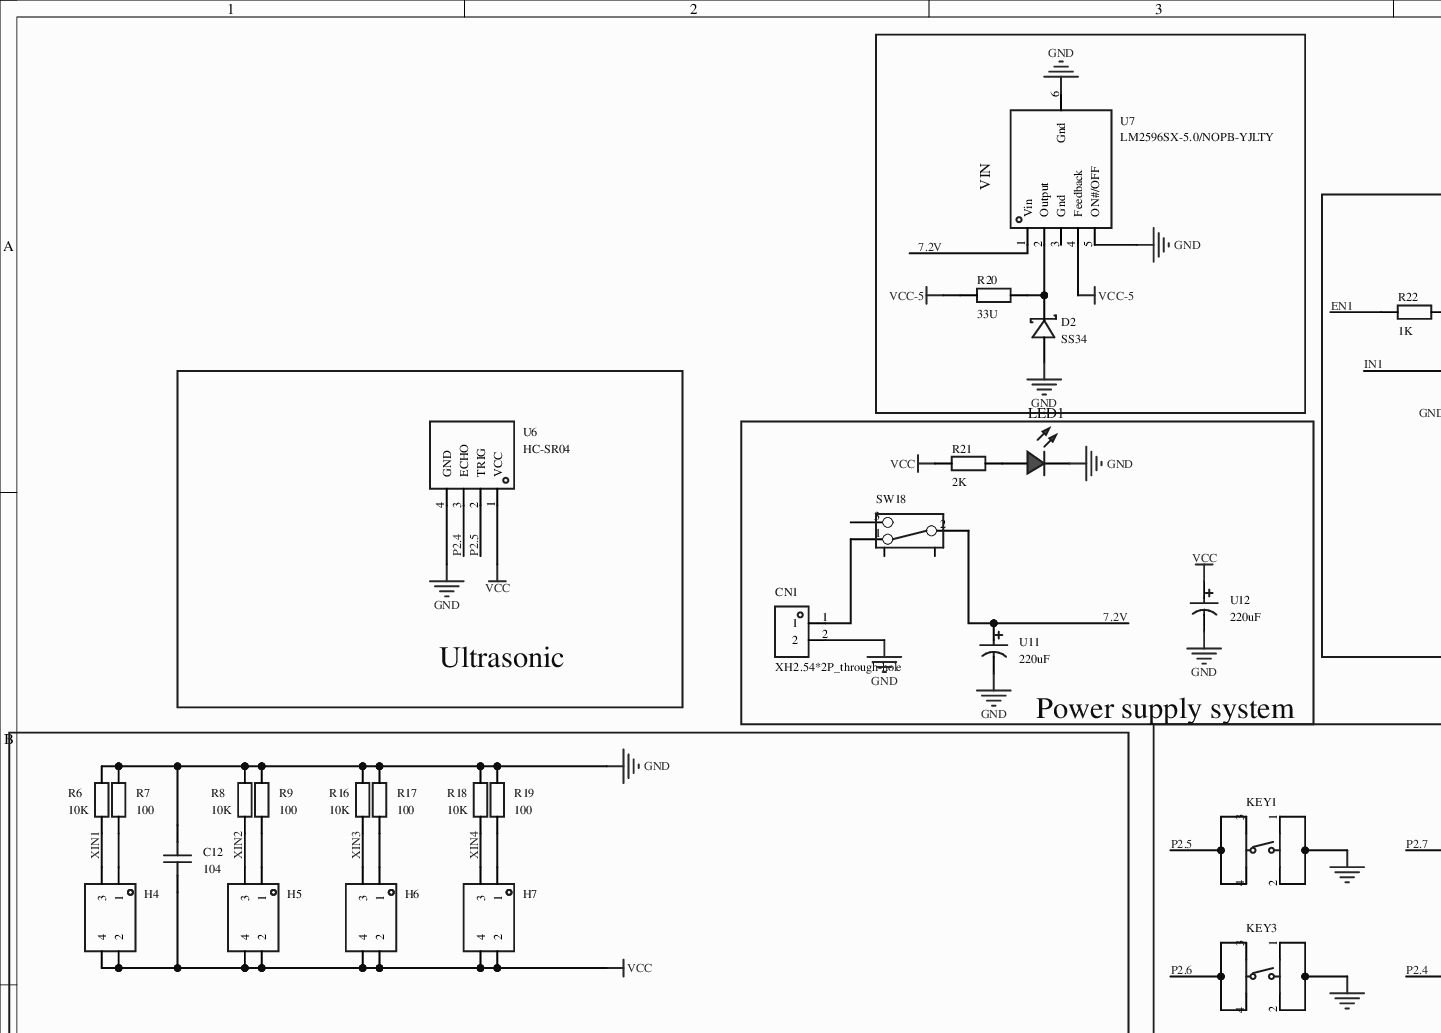
[diagram p0: MISC51732-3.schdoc, top left]
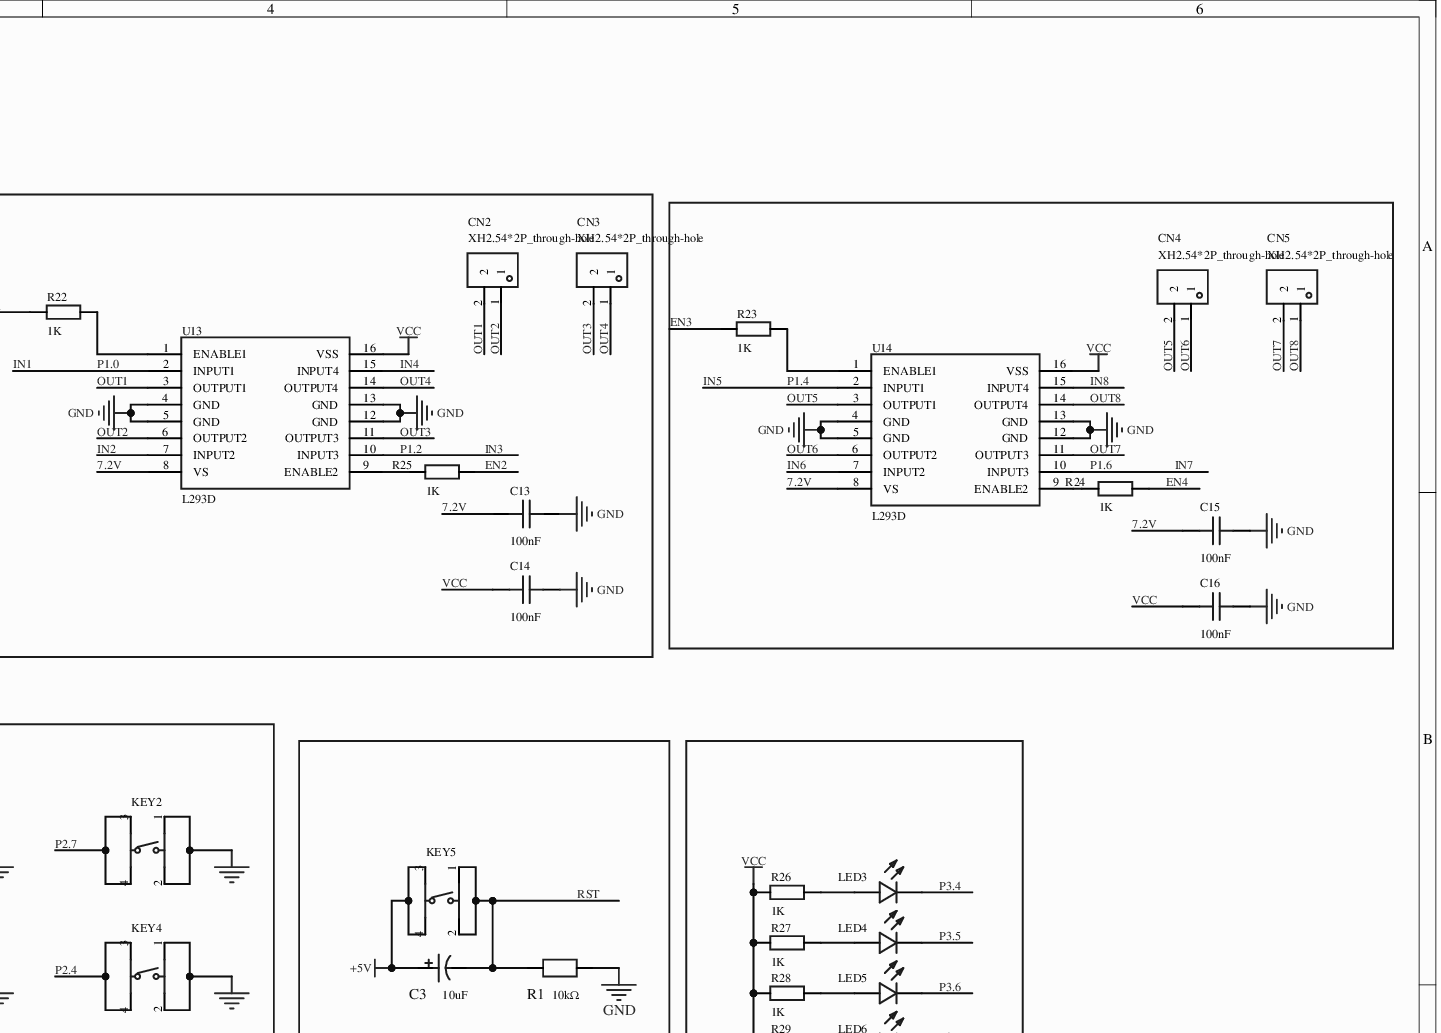
[diagram p1: MISC51732-3.schdoc, top right]
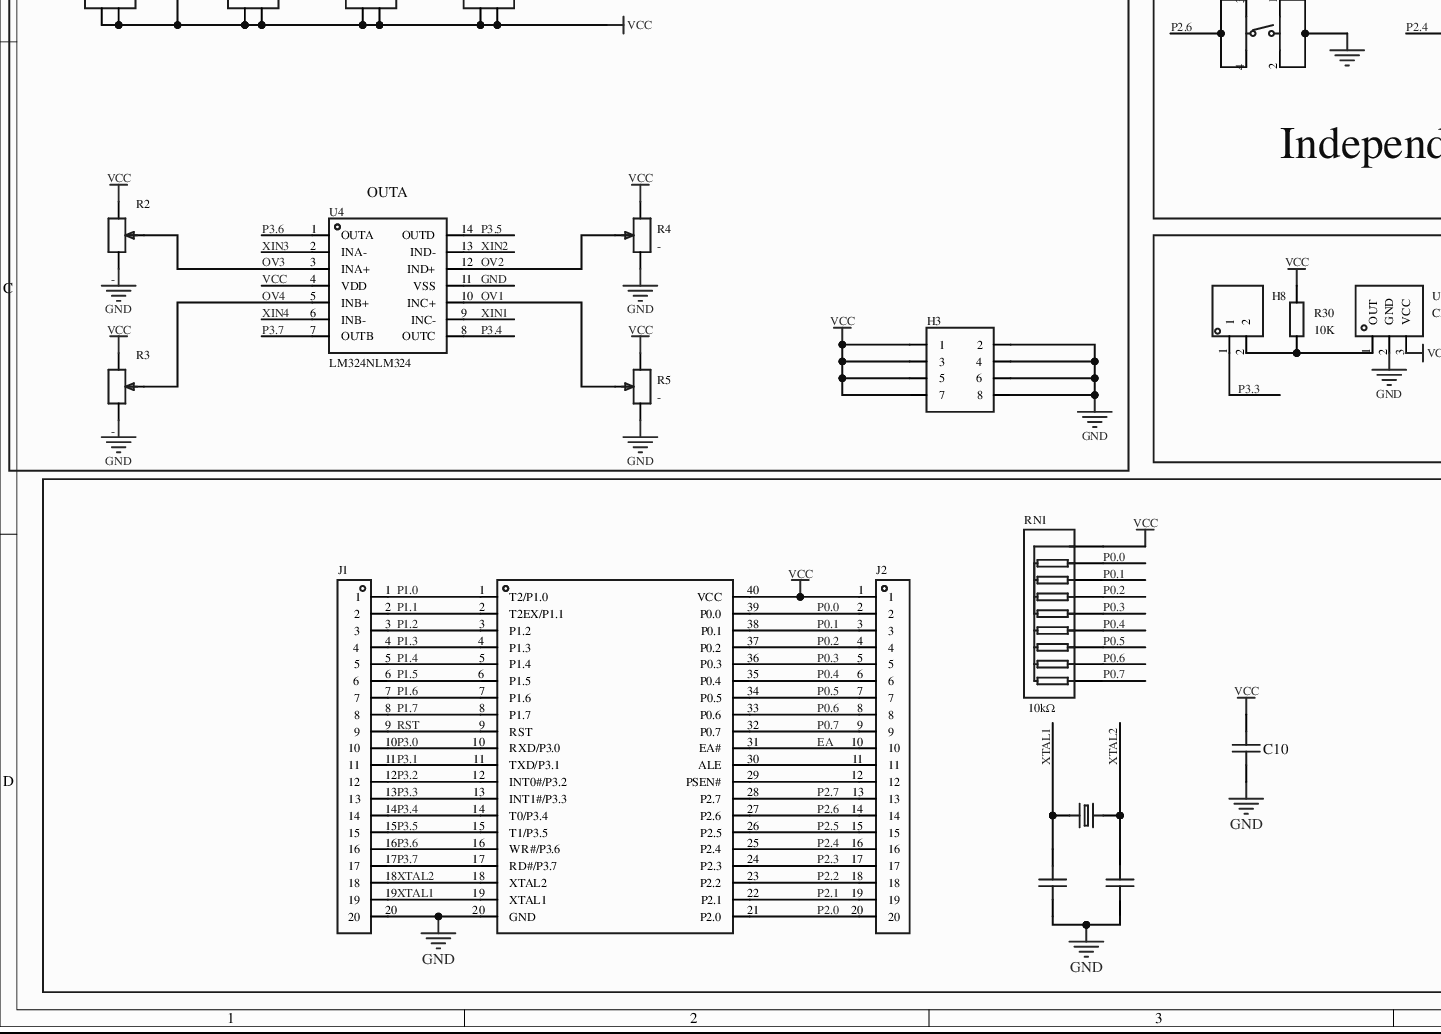
[diagram p2: MISC51732-3.schdoc, bottom left]
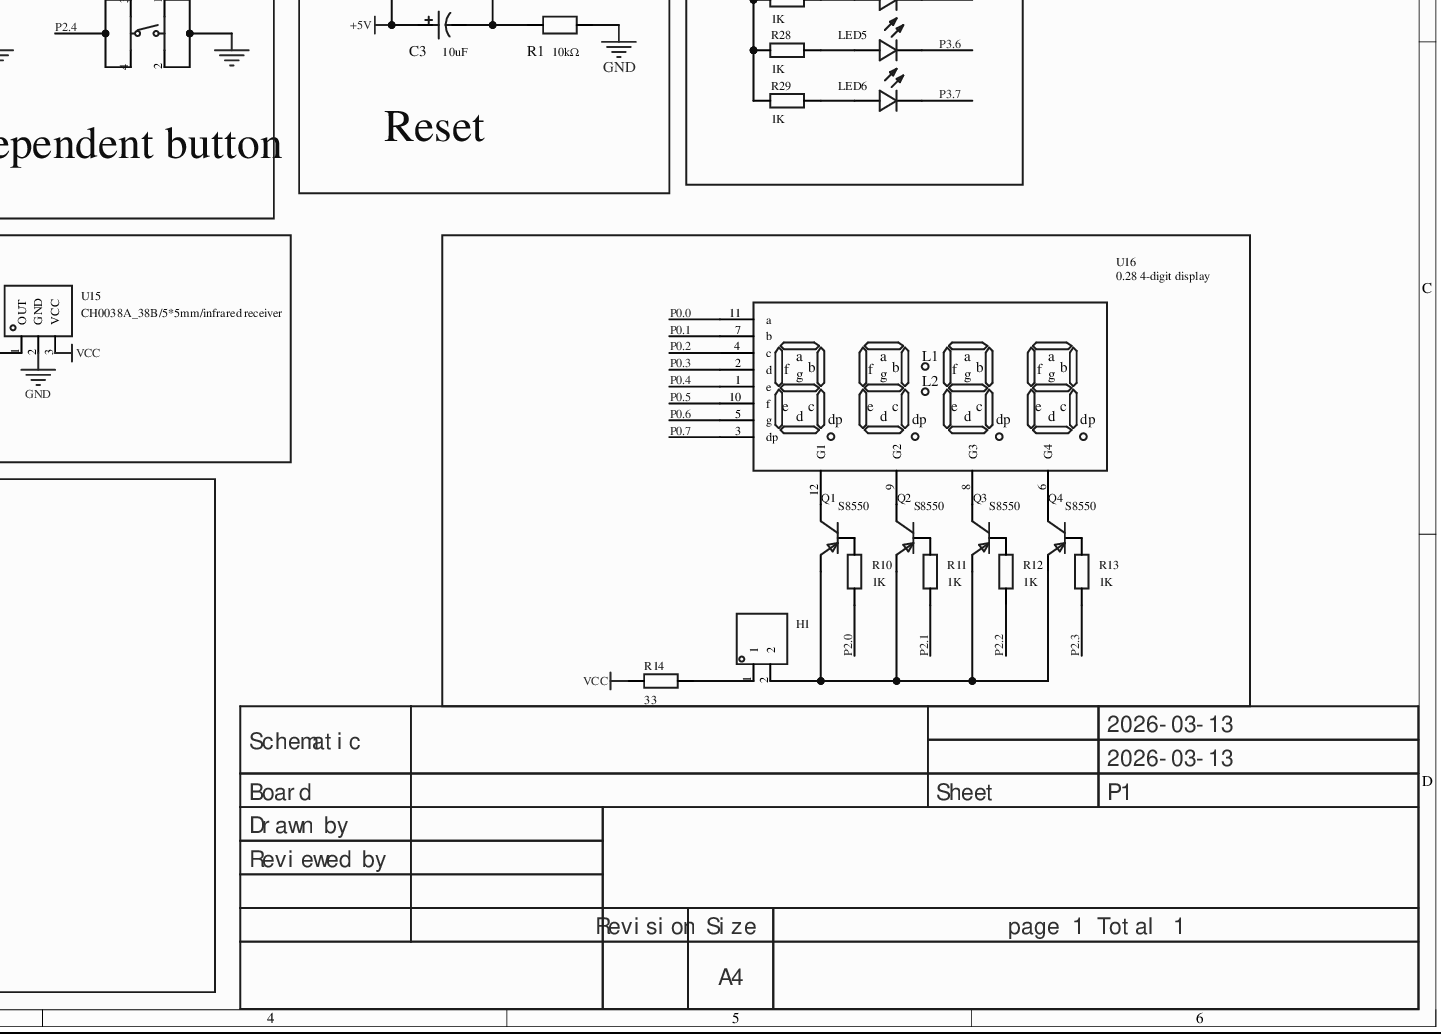
[diagram p3: MISC51732-3.schdoc, bottom right]
# Altium project MISC51732-2.PrjPcb
1 sheet, 80 parts. Net scope: global (net labels, ports and power ports of the same name join across sheets).
Board file: MISC51732.pcbdoc

## Sheet MISC51732-3.schdoc
size 420 x 297 mm; Version: V1.0; @Project Name: MISC51732; @Update Date: 2026-03-13; @Create Date: 2026-03-13; @Board Name: MISC51732; @Create Time: 21:41:42; @Page Count: 1; @Page No: 1; @Schematic Name: MISC51732; @Update Time: 21:41:42; Size: A4

### Parts
C1  (no value)  [CAP-TH_L5.0-W2.5-P5.08-D0.7]
C2  (no value)  [CAP-TH_L5.0-W2.5-P5.08-D0.7]
C3  value 10uF  [CAP-TH_BD5.0-P2.00-D0.8-FD]
C10  (no value)  [CAP-TH_L5.0-W2.5-P5.00-D1.0]
C12  104  [C0603]
C13  100nF  [C0603]
C14  100nF  [C0603]
C15  100nF  [C0603]
C16  100nF  [C0603]
CN1  XH2.54*2P_through-hole  [CONN-TH_2P-P2.50-XH2.54-2P]
CN2  XH2.54*2P_through-hole  [CONN-TH_2P-P2.50-XH2.54-2P]
CN3  XH2.54*2P_through-hole  [CONN-TH_2P-P2.50-XH2.54-2P]
CN4  XH2.54*2P_through-hole  [CONN-TH_2P-P2.50-XH2.54-2P]
CN5  XH2.54*2P_through-hole  [CONN-TH_2P-P2.50-XH2.54-2P]
D2  SS34  [SMA_L4.3-W2.6-LS5.0-RD]
H1  (no value)  [HDR-TH_2P-P2.54-V-M-1]
H3  (no value)  [HDR-TH_8P-P2.54-V-F-R2-C4-S2.54-1]
H4  (no value)  [HDR-TH_4P-P2.54-V-F-R2-C2-S2.54]
H5  (no value)  [HDR-TH_4P-P2.54-V-F-R2-C2-S2.54]
H6  (no value)  [HDR-TH_4P-P2.54-V-F-R2-C2-S2.54]
H7  (no value)  [HDR-TH_4P-P2.54-V-F-R2-C2-S2.54]
H8  (no value)  [HDR-TH_2P-P2.54-V-M-1]
J1  (no value)  [HDR-TH_20P-P2.54-V-M-1]
J2  (no value)  [HDR-TH_20P-P2.54-V-M-1]
KEY1  UK-B0202-G5-160  [SW-TH_4P-L6.0-W6.0-P4.50-LS6.5]  (value not drawn)
KEY2  UK-B0202-G5-160  [SW-TH_4P-L6.0-W6.0-P4.50-LS6.5]  (value not drawn)
KEY3  UK-B0202-G5-160  [SW-TH_4P-L6.0-W6.0-P4.50-LS6.5]  (value not drawn)
KEY4  UK-B0202-G5-160  [SW-TH_4P-L6.0-W6.0-P4.50-LS6.5]  (value not drawn)
KEY5  UK-B0202-G5-160  [SW-TH_4P-L6.0-W6.0-P4.50-LS6.5]  (value not drawn)
LED1  (no value)  [LED_0603]
LED3  (no value)  [LED-TH_BD3.0-P2.54-FD]
LED4  (no value)  [LED-TH_BD3.0-P2.54-FD]
LED5  (no value)  [LED-TH_BD3.0-P2.54-FD]
LED6  (no value)  [LED-TH_BD3.0-P2.54-FD]
Q1  S8550  [SOT-23-3_L2.9-W1.6-P1.90-LS2.8-BR]
Q2  S8550  [SOT-23-3_L2.9-W1.6-P1.90-LS2.8-BR]
Q3  S8550  [SOT-23-3_L2.9-W1.6-P1.90-LS2.8-BR]
Q4  S8550  [SOT-23-3_L2.9-W1.6-P1.90-LS2.8-BR]
R1  value 10kΩ  [RES-TH_BD2.4-L6.3-P10.30-D0.6]
R2  -  [RES-ADJ-TH_3362P]
R3  -  [RES-ADJ-TH_3362P]
R4  -  [RES-ADJ-TH_3362P]
R5  -  [RES-ADJ-TH_3362P]
R6  10K  [R0603]
R7  100  [R0603]
R8  10K  [R0603]
R9  100  [R0603]
R10  1K  [R0603]
R11  1K  [R0603]
R12  1K  [R0603]
R13  1K  [R0603]
R14  33  [R0603]
R16  10K  [R0603]
R17  100  [R0603]
R18  10K  [R0603]
R19  100  [R0603]
R20  33U  [R0603]
R21  2K  [R0603]
R22  1K  [R0603]
R23  1K  [R0603]
R24  1K  [R0603]
R25  1K  [R0603]
R26  1K  [R0603]
R27  1K  [R0603]
R28  1K  [R0603]
R29  1K  [R0603]
R30  10K  [R0603]
RN1  value 10kΩ  [RES-ARRAY-TH_9P-P2.54-D1.0]
SW18  (no value)  [拨动开关]
U1  (no value)  [DIP-40_L52.0-W13.7-P2.54-LS15.2-BL]
U4  LM324NLM324  [SOP-14_L8.6-W3.9-P1.27-LS6.0-BL]
U6  HC-SR04  [TH_HC-SR04V]
U7  LM2596SX-5.0/NOPB-YJLTY  [TO-263-5_L10.0-W8.4-P1.70-LS15.3-BR]
U11  220uF  [CAP-SMD_BD6.3-L6.6-W6.6-LS7.2-FD]
U12  220uF  [CAP-SMD_BD6.3-L6.6-W6.6-LS7.2-FD]
U13  L293D  [DIP-16_L20.0-W6.4-P2.54-LS7.6-BL]
U14  L293D  [DIP-16_L20.0-W6.4-P2.54-LS7.6-BL]
U15  CH0038A_38B/5*5mm/infrared receiver  [OPTO-SMD_CH0038A_38B]
U16  0.28 4-digit display  [LED-SEG-TH_12P-L32.1-W10.0-P12.7-S7.62-BL]
X1  (no value)  [HC-49US_L11.5-W4.5-P4.88]

### Blocks framed on the sheet
Ultrasonic: U6
Power supply system: CN1 LED1 R21 SW18 U11 U12
Independent button: KEY1-KEY4
Reset: C3 KEY5 R1

### Nets
+5V: C3.1 KEY5.3 KEY5.4
GND: C1.2 C2.2 C10.1 C12.2 C13.2 C14.2 C15.2 C16.2 CN1.2 D2.2(A) H3.2 H3.4 H3.6 H3.8 J1.20 KEY1.1 KEY1.2 KEY2.1 KEY2.2 KEY3.1 KEY3.2 KEY4.1 KEY4.2 LED1.1(C) R1.2 R2.3 R3.3 R4.3 R5.3 R6.2 R7.2 R8.2 R9.2 R16.2 R17.2 R18.2 R19.2 U1.20(GND) U4.11(VSS) U6.4(GND) U7.5(ON#/OFF) U7.6(Gnd) U11.2 U12.2 U13.4(GND) U13.5(GND) U13.12(GND) U13.13(GND) U14.4(GND) U14.5(GND) U14.12(GND) U14.13(GND) U15.2(GND)
VCC: C10.2 C12.1 C14.1 C16.1 H3.1 H3.3 H3.5 H3.7 H4.2 H4.4 H5.2 H5.4 H6.2 H6.4 H7.2 H7.4 J2.1 R2.1 R3.1 R4.1 R5.1 R14.1 R21.1 R26.1 R27.1 R28.1 R29.1 R30.2 RN1.1 U1.40(VCC) U4.4(VDD) U6.1(VCC) U12.1 U13.16(VSS) U14.16(VSS) U15.3(VCC)
VCC-5: R20.1 U7.4(Feedback)
7.2V: C13.1 C15.1 SW18.2 U7.1(Vin) U11.1 U13.8(VS) U14.8(VS)
EA: J2.10 U1.31(EA#)
EN1: R22.1
EN2: R25.2
EN3: R23.1
EN4: R24.2
IN1: J1.1 U1.1(T2/P1.0) U13.2(INPUT1)  [also labelled P1.0]
IN2: U13.7(INPUT2)
IN3: J1.3 U1.3(P1.2) U13.10(INPUT3)  [also labelled P1.2]
IN4: U13.15(INPUT4)
IN5: J1.5 U1.5(P1.4) U14.2(INPUT1)  [also labelled P1.4]
IN6: U14.7(INPUT2)
IN7: J1.7 U1.7(P1.6) U14.10(INPUT3)  [also labelled P1.6]
IN8: U14.15(INPUT4)
OUT1: CN2.2 U13.3(OUTPUT1)
OUT2: CN2.1 U13.6(OUTPUT2)
OUT3: CN3.2 U13.11(OUTPUT3)
OUT4: CN3.1 U13.14(OUTPUT4)
OUT5: CN4.2 U14.3(OUTPUT1)
OUT6: CN4.1 U14.6(OUTPUT2)
OUT7: CN5.2 U14.11(OUTPUT3)
OUT8: CN5.1 U14.14(OUTPUT4)
OV1: R5.2 U4.10(INC+)
OV2: R4.2 U4.12(IND+)
OV3: R2.2 U4.3(INA+)
OV4: R3.2 U4.5(INB+)
P0.0: J2.2 RN1.2 U1.39(P0.0) U16.11(a)
P0.1: J2.3 RN1.3 U1.38(P0.1) U16.7(b)
P0.2: J2.4 RN1.4 U1.37(P0.2) U16.4(c)
P0.3: J2.5 RN1.5 U1.36(P0.3) U16.2(d)
P0.4: J2.6 RN1.6 U1.35(P0.4) U16.1(e)
P0.5: J2.7 RN1.7 U1.34(P0.5) U16.10(f)
P0.6: J2.8 RN1.8 U1.33(P0.6) U16.5(g)
P0.7: J2.9 RN1.9 U1.32(P0.7) U16.3(dp)
P1.1: J1.2 U1.2(T2EX/P1.1)
P1.3: J1.4 U1.4(P1.3)
P1.5: J1.6 U1.6(P1.5)
P1.7: J1.8 U1.8(P1.7)
P2.0: J2.20 R10.1 U1.21(P2.0)
P2.1: J2.19 R11.1 U1.22(P2.1)
P2.2: J2.18 R12.1 U1.23(P2.2)
P2.3: J2.17 R13.1 U1.24(P2.3)
P2.4: J2.16 KEY4.3 KEY4.4 U1.25(P2.4) U6.3(ECHO)
P2.5: J2.15 KEY1.3 KEY1.4 U1.26(P2.5) U6.2(TRIG)
P2.6: J2.14 KEY3.3 KEY3.4 U1.27(P2.6)
P2.7: J2.13 KEY2.3 KEY2.4 U1.28(P2.7)
P3.0: J1.10 U1.10(RXD/P3.0)
P3.1: J1.11 U1.11(TXD/P3.1)
P3.2: J1.12 U1.12(INT0#/P3.2)
P3.3: H8.1 J1.13 U1.13(INT1#/P3.3)
P3.4: J1.14 LED3.2(K) U1.14(T0/P3.4) U4.8(OUTC)
P3.5: J1.15 LED4.2(K) U1.15(T1/P3.5) U4.14(OUTD)
P3.6: J1.16 LED5.2(K) U1.16(WR#/P3.6) U4.1(OUTA)
P3.7: J1.17 LED6.2(K) U1.17(RD#/P3.7) U4.7(OUTB)
RST: C3.2 J1.9 KEY5.1 KEY5.2 R1.1 U1.9(RST)
XIN1: H4.3 R6.1 U4.9(INC-)
XIN2: H5.3 R8.1 U4.13(IND-)
XIN3: H6.3 R16.1 U4.2(INA-)
XIN4: H7.3 R18.1 U4.6(INB-)
XTAL1: C1.1 J1.19 U1.19(XTAL1) X1.2
XTAL2: C2.1 J1.18 U1.18(XTAL2) X1.1
NetCN1_1: CN1.1 SW18.1
NetD2_1: D2.1(K) R20.2 U7.2(Output)
NetH1_1: H1.1 R14.2
NetH1_2: H1.2 Q1.2 Q2.2 Q3.2 Q4.2
NetH4_1: H4.1 R7.1
NetH5_1: H5.1 R9.1
NetH6_1: H6.1 R17.1
NetH7_1: H7.1 R19.1
NetH8_2: H8.2 R30.1 U15.1(OUT)
NetJ2_11: J2.11 U1.30(ALE)
NetJ2_12: J2.12 U1.29(PSEN#)
NetLED1_2: LED1.2(A) R21.2
NetLED3_1: LED3.1(A) R26.2
NetLED4_1: LED4.1(A) R27.2
NetLED5_1: LED5.1(A) R28.2
NetLED6_1: LED6.1(A) R29.2
NetQ1_1: Q1.1 R10.2
NetQ1_3: Q1.3 U16.12(G1)
NetQ2_1: Q2.1 R11.2
NetQ2_3: Q2.3 U16.9(G2)
NetQ3_1: Q3.1 R12.2
NetQ3_3: Q3.3 U16.8(G3)
NetQ4_1: Q4.1 R13.2
NetQ4_3: Q4.3 U16.6(G4)
NetR22_2: R22.2 U13.1(ENABLE1)
NetR23_2: R23.2 U14.1(ENABLE1)
NetR24_1: R24.1 U14.9(ENABLE2)
NetR25_1: R25.1 U13.9(ENABLE2)

Not connected (* = marked no-connect by the designer): SW18 3 4 5; U7 3(Gnd)

### Notes on the sheet
- 2026-03-13
- Schematic
- Board
- Sheet
- P1
- Drawn by
- Reviewed by
- Revision
- Size
- A4
- page 1 Total 1

### Library data of the parts
C1 C2 = CC1H330JC74DCH4B10MN: Capacitance:33pF;Tolerance:±5%;Rated voltage:50V;Temperature coefficient:NP0;Lead pitch:5.08mm;Body diameter:4.7mm;Body thickness:2.2mm;; Manufacturer: Dersonic(德尔创); 3D Model: 3d005bb2736f4b028b929daf59d2a504; 3D Model Transform: 222.8342,98.419,0,0,0,0,0,0,-118.11; Value: 33pF; Tolerance: ±5%; Voltage Rated: 50V; Temperature Coefficient: NP0; φD: 4.7mm; Body Thickness: 2.2mm; AddInBom: yes; ModelName: CAP-TH_L5.0-W2.5-P5.08; Symbol: CC1H330JC74DCH4B10MN; Device: CC1H330JC74DCH4B10MN; LCSC Part Name: 33pF ±5% 50V; Supplier Part: C254101; Manufacturer Part: CC1H330JC74DCH4B10MN; Supplier Footprint: 径向引线,P=5.08mm; JLCPCB Part Class: Extended Part; Datasheet: example.com/upload/public/pdf/source/20200826/C254101_16B526CCB578B7B7F57569795E2616C1.pdf; Supplier: LCSC; Lead Spacing: 5.08mm; ConvertToPcb: yes; FootprintName: CAP-TH_L5.0-W2.5-P5.08-D0.7
C3 = KM106M050D11RR0VH2FP0: Capacitance:10uF;Tolerance:±20%;Rated voltage:50V;Body diameter:5mm;Body length:11mm;Lead pitch:2mm;Operating life:1000hrs@105;; Manufacturer: CX(承兴); Symbol: 10uF 50V 5*11; 3D Model: edeeed87cbc746108d01291548c38636; 3D Model Transform: 197.1,196.7,0,180,0,180,0,0,275.6; Tolerance: ±20%; Rated Voltage: 50V; φD: 5mm; L: 11mm; AddInBom: yes; ModelName: CAP-TH_D5.0H7.0P2.0; Device: KM106M050D11RR0VH2FP0; Lifetime @ Temp: 1000hrs@105; LCSC Part Name: 10uF ±20% 50V; Supplier Part: C43345; Manufacturer Part: KM106M050D11RR0VH2FP0; Supplier Footprint: 径向引线,5x11mm; JLCPCB Part Class: Extended Part; Datasheet: example.com/upload/public/pdf/source/20211027/06D6BA3719C264B639DC286D935D03EA.pdf; Supplier: LCSC; Lead Spacing: 2mm; ConvertToPcb: yes; FootprintName: CAP-TH_BD5.0-P2.00-D0.8-FD
C10 = CC1H104MC1FD3F6C10MF: Capacitance:100nF;Tolerance:±20%;Rated voltage:50V;Temperature coefficient:Y5V;Lead pitch:5.08mm;Body diameter:6mm;Body thickness:2.2mm;; Manufacturer: Dersonic(德尔创); 3D Model: 08e3d7481fc7486bb1b263873f51e1e1; 3D Model Transform: 224.7,98.4,0,0,0,0,0,0,-137.8; Value: 100nF; Tolerance: ±20%; Voltage Rated: 50V; Temperature Coefficient: Y5V; φD: 6mm; Body Thickness: 2.2mm; AddInBom: yes; ModelName: CAP-TH_BD5.0-W2.5-P5.08; Symbol: CC1H104MC1FD3F6C10MF; Device: CC1H104MC1FD3F6C10MF; LCSC Part Name: 100nF ±20% 50V; Supplier Part: C254085; Manufacturer Part: CC1H104MC1FD3F6C10MF; Supplier Footprint: 径向引线,P=5.08mm; JLCPCB Part Class: Extended Part; Datasheet: example.com/upload/public/pdf/source/20200826/C254085_159DD65BF32BF11C9168D341BCE23E6F.pdf; Supplier: LCSC; Lead Spacing: 5.08mm; ConvertToPcb: yes; FootprintName: CAP-TH_L5.0-W2.5-P5.00-D1.0
C12-C16 = CAP_0603: Symbol: Capacitance; ConvertToPcb: yes; ModelId: ac125912035d415993ca9572d50418b10819f05c4eef4c71ace90d822a990e87; ModelName: C0603_L1.6-W0.8-H0.8; ModelTransform: 62.992,31.496,0,0,0,0,0,0,0; Device: CAP_0603; AddInBom: yes; Supplier Footprint: 0603; FootprintName: C0603
  C12: Value: 104
  C13-C16: Value: 100nF
CN1-CN5 = XH2.54*2P_直插: AddInBom: yes; ModelId: 325c595e30db4df8abe76612dd40b0fa0819f05c4eef4c71ace90d822a990e87; ModelTransform: 295.275,228.346,0,180,0,0,-0.002,-20.079,-137.795; Symbol: XH2.54*2P_through-hole; Device: XH2.54*2P_through-hole; LCSC Part Name: XH2.54*2P_直插; SupplierPart: C9900008615; ManufacturerPart: XH2.54*2P_直插; Supplier Footprint: XH2.54_2P; JLCPCB Part Class: Extended Part; Supplier: LCSC; ConvertToPcb: yes; FootprintName: CONN-TH_2P-P2.50-XH2.54-2P; ModelName: CONN-TH_2P-P2.50-XH2.54-2P
D2 = SS34: Symbol: SS34_C9900023345; AddInBom: yes; ModelId: 8d2dd2e50a3a4b27821fa63d469a8f110819f05c4eef4c71ace90d822a990e87; ModelTransform: 196.85,102.362,0,0,0,0,0,0,0; Device: SS34; LCSC Part Name: SS34; SupplierPart: C9900023345; ManufacturerPart: SS34; Supplier Footprint: SMA,DO-214AC; JLCPCB Part Class: Extended Part; Supplier: LCSC; ConvertToPcb: yes; FootprintName: SMA_L4.3-W2.6-LS5.0-RD; ModelName: SMA_L4.3-W2.6-LS5.0-RD
H1 H8 = HDR-M_2.54_1x2P: Symbol: 210S-1*2P L=11.6MMGold-plated black; ConvertToPcb: yes; ModelId: 79b2e9f2d70a4d68a1b7098f27c6d4c50819f05c4eef4c71ace90d822a990e87; ModelName: HDR-M-2.54_1x2; ModelTransform: 200,100,0,0,0,0,0,0,-118.11; Device: HDR-M_2.54_1x2P; AddInBom: yes; SupplierPart: C124375; Supplier Footprint: 插件; FootprintName: HDR-TH_2P-P2.54-V-M-1
H3 = HDR-F_2.54_2x4: Symbol: HDR-F-2.54_2x4; ConvertToPcb: yes; ModelId: 64729f32a5874cf59655d275a66f10500819f05c4eef4c71ace90d822a990e87; ModelName: HDR2.54-F-LI-2X4P; ModelTransform: 399.999,200,0,0,0,0,0,0,-118.11; Device: HDR-F_2.54_2x4; AddInBom: yes; SupplierPart: C92271; Supplier Footprint: 插件; FootprintName: HDR-TH_8P-P2.54-V-F-R2-C4-S2.54-1
H4-H7 = HDR-F_2.54_2x2: Symbol: HDR-F-2.54_2x2; ConvertToPcb: yes; ModelId: 870c884146ee4765973edc845f10b7af0819f05c4eef4c71ace90d822a990e87; ModelName: HDR-TH_4P-P2.54-F-LI-2X2P; ModelTransform: 215.7476,196.85,0,0,0,0,0,0,-118.11; Device: HDR-F_2.54_2x2; AddInBom: yes; SupplierPart: C92273; Supplier Footprint: 插件; FootprintName: HDR-TH_4P-P2.54-V-F-R2-C2-S2.54
J1 J2 = 2.54-1*20P直针: Pitch:2.54mm;Total pin count:20;Rows:1;Pin structure:-;Row spacing:-;Mounting type:through-hole;Round/square pin:-;Rated current:-;Rated voltage:-;Mating pin length:-;Plastic height:-;Contact material:brass;Contact plating:-;Colour:black;; Manufacturer: BOOMELE(博穆精密); Symbol: Header-Male-2.54_1x20; Device: 2.54-1*20P straight pin; 3D Model: f68709be121d406db68b06f32a595389; 3D Model Transform: 2000,100,0,0,0,0,0,2.5,-118.1; Pitch: 2.54mm; AddInBom: yes; ModelName: HDR-M-2.54_1x20; LCSC Part Name: 2.54mm; Supplier Part: C50981; Manufacturer Part: 2.54-1*20P直针; Supplier Footprint: 插件,P=2.54mm; JLCPCB Part Class: Extended Part; Datasheet: example.com/upload/public/pdf/source/20151109/1457707571495.pdf; Supplier: LCSC; Number of Pins: 20; Number of Rows: 1; Pin Structure: -; Row Spacing: -; Mounting Type: Through-hole; Circluar Pins/Square Pins: -; Current Rating (Max): -; Voltage Rating (Max): -; Length of Mating Pin: -; Insulation Height: -; Contact Material: Brass; Contact Plating: -; Color: Black; ConvertToPcb: yes; FootprintName: HDR-TH_20P-P2.54-V-M-1
KEY1-KEY5 = UK-B0202-G5-160: Contact current:50mA;Rated voltage (DC):12V;Insulation resistance:100MΩ;Circuit:SPST;Mounting type:through-hole;Button shape:round button;Button/cap colour:black;With lamp:no;Actuating force:160gf@±50gf;Mechanical life:100000;Operating temperature:-20~+70;Pin style:PC pin;Switch length:6mm;Switch width:6mm;Switch height:5mm;With bracket:no;; Manufacturer: USAKRO(美韩); 3D Model: 20eee248bc684ccd8cbdbb1d0d91ec6f; 3D Model Transform: 236.22,323.03,0,90,0,0,0,0,-137.795; Contact Current: 50mA; Voltage Rating (DC): 12V; Insulation Resistance: 100MΩ; Circuit: SPST; Actuator/Cap Color: Black; With Lamp: No; Mechanical Life: 100000; Pin Style: PC pin; Switch Length: 6mm; Switch Height: 5mm; AddInBom: yes; ModelName: SW-TH_4P-L6.0-W6.0-H5.0-LS6.5-P4.50; Symbol: UK-B0202-G5-160; Device: UK-B0202-G5-160; Operating Temperature: -20~+70; LCSC Part Name: 6*6*5 160gf; Supplier Part: C620202; Manufacturer Part: UK-B0202-G5-160; Supplier Footprint: 插件; JLCPCB Part Class: Extended Part; Datasheet: example.com/upload/public/pdf/source/20200616/C620202_665E30154320151E26EE2009FF61E3DC.pdf; Supplier: LCSC; Mounting Style: Through-hole; Actuator Style: Round button; Operating Force: 160gf@±50gf; Switch Width: 6mm; Strike Gundam: No; ConvertToPcb: yes; FootprintName: SW-TH_4P-L6.0-W6.0-P4.50-LS6.5
LED1 = LED_0603-R: Symbol: LED_R; Convert to PCB: yes; 3D Model: dd8257b0d61a4cd7b68939a056e080950819f05c4eef4c71ace90d822a990e87; 3D Model Transform: 58.72,29.4,22.03,0,0,0,0,0,0; ModelName: LED-0603_R; Device: LED_0603-R; Add into BOM: yes; Supplier Footprint: 0603; FootprintName: LED_0603
LED3-LED6 = 204-10SURD/S530-A3-L: Emitted colour:red;Diode configuration:-;Lens colour:diffused red;Dominant wavelength:624nm;Peak wavelength:632nm;Colour temperature:-;Luminous flux (25):-;Test current:20mA;Forward voltage (VF):2V;Luminous intensity:80mcd;Power:60mW;Viewing angle:40°;Mounting type:-;Operating temperature:-40~+85;; Manufacturer: EVERLIGHT(台湾亿光); 3D Model: a497c992633541038a38947cdc58012f; 3D Model Transform: 141.274,153.327,0,0,0,0,-5.984,0,-137.795; Dominant Wavelength: 624nm; Peak Wavelength: 632nm; Forward Current: 20mA; Forward Voltage (VF): 2V; Luminous Intensity: 80mcd; Power Dissipation: 60mW; Viewing Angle: 40°; AddInBom: yes; ModelName: LED-TH-3mm_R; Symbol: 204-10SURD/S530-A3-L; Device: 204-10SURD/S530-A3-L; Operating Temperature: -40~+85; LCSC Part Name: 红灯; Supplier Part: C99771; Manufacturer Part: 204-10SURD/S530-A3-L; Supplier Footprint: 插件,D=3mm; JLCPCB Part Class: Extended Part; Datasheet: example.com/upload/public/pdf/source/20170504/1493866972127.pdf; Supplier: LCSC; Emitted Color: Red; Diode Configuration: -; Lens Color: Diffused red; Color Temperature: -; Luminous Flux (@25℃): -; Mounting Sytle: -; ConvertToPcb: yes; FootprintName: LED-TH_BD3.0-P2.54-FD
Q1-Q4 = S8550(RANGE:120-200): Transistor type:PNP;Collector current (Ic):500mA;Collector-emitter breakdown voltage (Vceo):25V;Power dissipation (Pd):300mW;DC current gain (hFE):120@50mA,1V;; Manufacturer: CJ(江苏长电/长晶); Symbol: S8550_C105432; AddInBom: yes; ModelId: 89cb27a44ab2466697082bb9fd73a7d00819f05c4eef4c71ace90d822a990e87; ModelName: SOT-23-3L_L2.9-W1.6-H1.1-LS2.8-P0.95; ModelTransform: 114.173,110.236,0,90,0,0,0,0,0; type: PNP; Current - Collector(Ic): 500mA; Collector - Emitter Voltage VCEO: 25V; Pd - Power Dissipation: 300mW; Transition frequency(fT): 150MHz; Current - Collector Cutoff: 100nA; Vce Saturation(VCE(sat)): 600mV@500mA,50mA; Emitter-Base Voltage(Vebo): 5V; Device: S8550(RANGE:120-200); Manufacturer Part: S8550; LCSC Part Name: L档120-200 PNP 电流:0.5A 电压:25V; SupplierPart: C105432; Supplier Footprint: SOT-23; JLCPCB Part Class: Basic Part; Datasheet: example.com/datasheet/S8550(RANGE%253A120-200)/106647.html; Supplier: LCSC; ConvertToPcb: yes; FootprintName: SOT-23-3_L2.9-W1.6-P1.90-LS2.8-BR; DC Current Gain: 120@50mA,1V; Operating Temperature: -55℃~+150℃
R1 = RN 1/4W 10K F T/B A1: Resistor type:metal film resistor;Resistance:10kΩ;Tolerance:±1%;Power:250mW;Temperature coefficient:±50ppm/;Max working voltage:250V;Operating temperature range:-55~+125;; Manufacturer: Tyohm(幸亚电阻); Temperature Coefficient: ±50ppm/; 3D Model: 463263665006444ab7a47bd11b0cf956; 3D Model Transform: 427.165,94.32816,0,0,0,0,0,0,-196.85; Tolerance: ±1%; Power(Watts): 250mW; Overload Voltage (Max): 250V; AddInBom: yes; Symbol: RN 1/4W 10K F T/B A1; Device: RN 1/4W 10K F T/B A1; Operating Temperature Range: -55~+125; LCSC Part Name: 10kΩ ±1% 250mW; Supplier Part: C410695; Manufacturer Part: RN 1/4W 10K F T/B A1; Supplier Footprint: 轴向引线; JLCPCB Part Class: Extended Part; Datasheet: example.com/upload/public/pdf/source/20190808/C410695_F4C96186075092C4BC649A77CE7E5B2A.pdf; Supplier: LCSC; Type: Metal film resistor; ConvertToPcb: yes; FootprintName: RES-TH_BD2.4-L6.3-P10.30-D0.6; ModelName: RES-TH_BD2.4-L6.3-P10.30-D0.6
R2-R5 = 3362P-1-103_C5047: Resistance:-;Power:-;; AddInBom: yes; ModelId: b1c5cb968ae748a39271ba681de641230819f05c4eef4c71ace90d822a990e87; ModelName: 3362P; ModelTransform: 271.653,279.527,0,0,0,0,0,-49.803,-232.283; Symbol: 3362P-1-103; Device: 3362P-1-103_C5047; LCSC Part Name: 10KΩ; SupplierPart: C5047; ManufacturerPart: 3362P-1-103; Supplier Footprint: 3362P; JLCPCB Part Class: Extended Part; Supplier: LCSC; ConvertToPcb: yes; FootprintName: RES-ADJ-TH_3362P; Value: -; Rated Voltage: -; Power(Watts): -; Turns: -
R6-R14 R16-R30 = Res_0603: Symbol: Resistor; ConvertToPcb: yes; ModelId: fc143cca1e79419f9cd78b61e9279f080819f05c4eef4c71ace90d822a990e87; ModelTransform: 31.8897,63.7794,0,90,0,0,0,0,0; Device: Res_0603; AddInBom: yes; Supplier Footprint: 0603; FootprintName: R0603; ModelName: R0603
  R6 R8 R16 R18 R30: Value: 10K
  R7 R9 R17 R19: Value: 100
  R10-R13 R22-R29: Value: 1K
  R14: Value: 33
  R20: Value: 33U
  R21: Value: 2K
RN1 = A09-103JP: Resistance:10kΩ;Tolerance:±5%;Power per element:125mW;Temperature coefficient:±100ppm/;Number of resistors:8;Pin count:9;; Manufacturer: FH(风华); 3D Model: d106c67f29e14d8080ba548247a719a1; 3D Model Transform: 917.49722,118.11,0,0,0,0,0,0,-137.795; Tolerance: ±5%; Power(Watts): 125mW; Number of Resistors: 8; AddInBom: yes; ModelName: SIP-9_L22.8-W3.0-H8.5-P2.54; Symbol: A09-103JP; Device: A09-103JP; Temperature Coefficient: ±100ppm/; LCSC Part Name: 10kΩ ±5%; Supplier Part: C8692; Manufacturer Part: A09-103JP; Supplier Footprint: SIP-9-2.54mm; JLCPCB Part Class: Extended Part; Datasheet: example.com/upload/public/pdf/source/20140224/1457706855244.pdf; Supplier: LCSC; Number of Pins: 9; ConvertToPcb: yes; FootprintName: RES-ARRAY-TH_9P-P2.54-D1.0
SW18 = 拨动开关_正: Symbol: Toggle switch; Device: Toggle switch_upright; ConvertToPcb: yes; ModelId: 4321fe59a4074cbfb4989553f297c68f0819f05c4eef4c71ace90d822a990e87; ModelName: SW-TH_SS-12D02-VG4; ModelTransform: 370.09,208.7,472.35,0,0,0,0,0,-110; AddInBom: yes; Supplier Footprint: 插件; FootprintName: Toggle switch
U1 = STC89C52RC-40I-PDIP40: CPU core:51 series;Max CPU frequency:-;Operating voltage range:3.3V~5.5V;Internal oscillator:-;External clock frequency range:-;Program FLASH capacity:8KB;Total RAM:512Byte;EEPROM/data FLASH capacity:4KB;GPIO port count:35;ADC (units/channels/bits):-;DAC (units/channels/bits):-;(E)PWM (units/channels/bits):-;8-bit Timer count:-;16-bit Timer count:3;32-bit Timer count:-;Internal comparator count:-;U(S)ART count:1;I2C count:-;I2S count:-;(; Manufacturer: STC(宏晶); 3D Model: 16d4686a009b4ddca948f91eddb57b14; 3D Model Transform: 2059.1,615.7,0,0,0,0,0,0,-118.1; Program FLASH Size: 8KB; EEPROM/Data FLASH Size: 4KB; GPIO Ports Number: 35; 16Bit Timer Number: 3; U(S)ART Number: 1; Peripherals / Functions / Protocol Stacks: Watchdog; AddInBom: yes; ModelName: DIP-40_L52.3-W13.8-H4.0-LS15.24-P2.54; Symbol: STC89C52RC-40I; Device: STC89C52RC-40I-PDIP40; Operating Temperature Range: -40~+85; LCSC Part Name: STC89C52RC-40I-PDIP40; Supplier Part: C14022; Manufacturer Part: STC89C52RC-40I-PDIP40; Supplier Footprint: DIP-40; JLCPCB Part Class: Extended Part; Datasheet: example.com/upload/public/pdf/source/20210104/C14022_3E6032FDBB5DBC6F971AD019A8472F5B.pdf; Supplier: LCSC; CPU Core: 51 series; Maximum Frequency: -; Supply Voltage Range: 3.3V~5.5V; Internal Oscillator: -; External Clock Frequency Rang: -; RAM Size: 512Byte; ADC (Units/Channels/bits): -; DAC (Units/Channels/bits): -; (E)PWM (Units/Channels/bits): -; 8Bit Timer Number: -; 32Bit Timer Number: -; CMP Number: -; I2C Number: -; I2S Number: -; (Q)SPI Number: -; CAN Number: -; USB (H/D/OTG): -; ConvertToPcb: yes; FootprintName: DIP-40_L52.0-W13.7-P2.54-LS15.2-BL
U4 = LM324NLM324: AddInBom: yes; ModelId: 520b569c4a2341089bdfdd9bf52b86190819f05c4eef4c71ace90d822a990e87; ModelTransform: 339.763,236.22,0,0,0,0,0,0,0; Symbol: LM324NLM324; Device: LM324NLM324; LCSC Part Name: LM324NLM324; SupplierPart: C9900015726; ManufacturerPart: LM324NLM324; Supplier Footprint: SOP-14; JLCPCB Part Class: Extended Part; Supplier: LCSC; ConvertToPcb: yes; FootprintName: SOP-14_L8.6-W3.9-P1.27-LS6.0-BL; ModelName: SOP-14_L8.6-W3.9-P1.27-LS6.0-BL
U6 = HC-SR04: Manufacturer: Universal Microelectronics; AddInBom: yes; Symbol: HC-SR04; Device: HC-SR04; LCSC Part Name: HC-SR04; SupplierPart: C19857336; ManufacturerPart: HC-SR04; Supplier Footprint: -; JLCPCB Part Class: Extended Part; Datasheet: example.com/datasheet/HC-SR04/21184790.html; Supplier: LCSC; ConvertToPcb: yes; FootprintName: TH_HC-SR04V
U7 = LM2596SX-5.0/NOPB-YJLTY: AddInBom: yes; ModelId: fb036f748a274327bb376552b66e43ac0819f05c4eef4c71ace90d822a990e87; ModelTransform: 388.9756,661.416,0,90,0,0,-43.311,0,0; Symbol: LM2596SX-5.0/NOPB-YJLTY; Device: LM2596SX-5.0/NOPB-YJLTY; LCSC Part Name: LM2596SX-5.0/NOPB-YJLTY; SupplierPart: C9900002281; ManufacturerPart: LM2596SX-5.0/NOPB-YJLTY; Supplier Footprint: TO-263-5; JLCPCB Part Class: Extended Part; Supplier: LCSC; ConvertToPcb: yes; FootprintName: TO-263-5_L10.0-W8.4-P1.70-LS15.3-BR; ModelName: TO-263-5_L10.0-W8.4-P1.70-LS15.3-BR
U11 U12 = 220uF: AddInBom: yes; ModelId: 1f98774f34d342b59c9890c435f425a30819f05c4eef4c71ace90d822a990e87; ModelTransform: 283.464,259.842,0,180,0,0,0,0,0; Symbol: 220UF; Device: 220uF; LCSC Part Name: 220uF; SupplierPart: C2941234; ManufacturerPart: 220uF; Supplier Footprint: -SMD6.3/5.8; JLCPCB Part Class: Extended Part; Supplier: LCSC; ConvertToPcb: yes; FootprintName: CAP-SMD_BD6.3-L6.6-W6.6-LS7.2-FD; ModelName: CAP-SMD_BD6.3-L6.6-W6.6-LS7.2-FD
U13 U14 = L293D: Push-pull quad driver with diodes; Manufacturer: ST(意法半导体); AddInBom: yes; ModelId: 6857a51368f0401381488830b088717c0819f05c4eef4c71ace90d822a990e87; ModelName: DIP-16_L20.0-W6.4-H3.5-LS7.62-P2.54; ModelTransform: 787.4,311.8104,0,0,0,0,0,0,-125.984; Number of H-bridges: 2; Output Current: 600mA; Peak Current: 1.2A; Voltage - Supply: 4.5V~36V; Quiescent Current(Iq): 4mA; Symbol: L293D; Device: L293D; LCSC Part Name: 600mA 有刷直流电机驱动芯片 36V; SupplierPart: C12340; ManufacturerPart: L293D; Supplier Footprint: DIP-16; JLCPCB Part Class: Extended Part; Datasheet: example.com/datasheet/L293D/12963.html; Supplier: LCSC; ConvertToPcb: yes; FootprintName: DIP-16_L20.0-W6.4-P2.54-LS7.6-BL; Technology: -; Interface: -; RDS(on): -; Operating Temperature: -40℃~+150℃
U15 = CH0038A_38B/5*5mm/红外接收头: AddInBom: yes; ModelId: 949982936b78483193c03311dd1fda000819f05c4eef4c71ace90d822a990e87; ModelTransform: 157.48,255.905,0,0,0,0,0,108.386,0; Symbol: CH0038A_38B/5*5MM/infrared receiver; Device: CH0038A_38B/5*5mm/infrared receiver; LCSC Part Name: CH0038A_38B/5*5mm/红外接收头; SupplierPart: C9900013915; ManufacturerPart: CH0038A_38B/5*5mm/红外接收头; Supplier Footprint: CH0038A_38B/5*5mm/红外接收头; JLCPCB Part Class: Extended Part; Supplier: LCSC; ConvertToPcb: yes; FootprintName: OPTO-SMD_CH0038A_38B; ModelName: OPTO-SMD_CH0038A_38B
U16 = 0.28 4位 数码管: AddInBom: yes; ModelId: df5be79ee1d1492281092420f86215950819f05c4eef4c71ace90d822a990e87; ModelName: LED-SEG-TH_12P-L32.1-W10.0-H5.8-P2.54-S7.62; ModelTransform: 1263.77696,393.7,0,0,0,0,0,0,-137.795; Symbol: 0.28 4-digit display; Device: 0.28 4-digit display; LCSC Part Name: 0.28 4位 数码管; SupplierPart: C9900013351; ManufacturerPart: 0.28 4位 数码管; Supplier Footprint: DIP-12; JLCPCB Part Class: Extended Part; Supplier: LCSC; ConvertToPcb: yes; FootprintName: LED-SEG-TH_12P-L32.1-W10.0-P12.7-S7.62-BL
X1 = TAXD12M2GLFBET2T: Crystal type:-;Frequency:-;Frequency tolerance:-;Load capacitance:-;Operating temperature:-;; Manufacturer: TAE(雅晶鑫); Symbol: HC-49S12MHZ20PF30PPM; 3D Model: a8e34f6c394c4d60ace7720f62d1ccdf; 3D Model Transform: 432.5,177.2,0,0,0,0,0,0,-137.8; AddInBom: yes; ModelName: HC-49US_L11.0-W4.5-H3.5-P4.88; Device: TAXD12M2GLFBET2T; LCSC Part Name: HC-49S 12MHz 20pF 30PPM; Supplier Part: C127674; Manufacturer Part: TAXD12M2GLFBET2T; Supplier Footprint: HC-49S-2P; JLCPCB Part Class: Extended Part; Datasheet: example.com/upload/public/pdf/source/20170914/C127674_1505359414286967688.pdf; Supplier: LCSC; Crystal Type: -; Value: -; Frequency Tolerance: -; Load Capacitance: -; Operating Temperature: -; ConvertToPcb: yes; FootprintName: HC-49US_L11.5-W4.5-P4.88